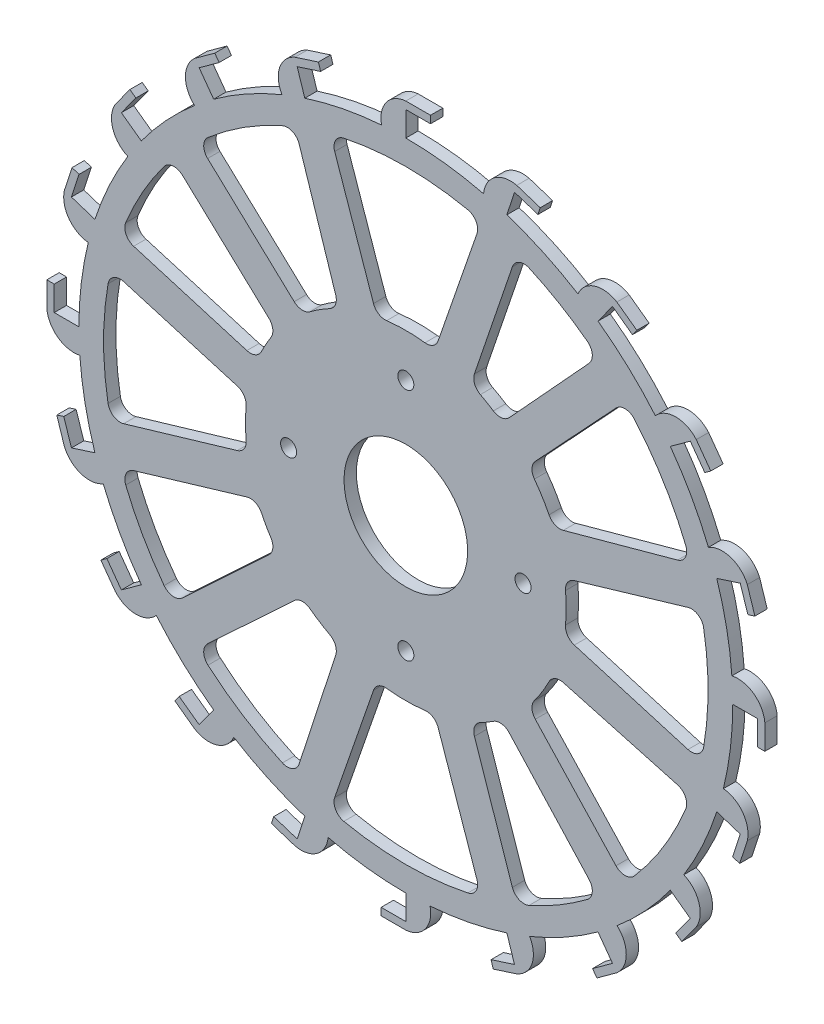
SolidWorks part; units mm, degrees
material "Q235A"
ref_plane "前视基准面" through (0, 0, 0) normal (0, 0, 1) x (1, 0, 0)
ref_plane "上视基准面" through (0, 0, 0) normal (0, 1, 0) x (1, 0, 0)
ref_plane "右视基准面" through (0, 0, 0) normal (1, 0, 0) x (0, 0, -1)
sketch "草图1" plane through (0, 0, 0) normal (0, 0, 1) x (1, 0, 0)
  line B0 (115.4655, -40.9141) -> (25.2954, -16.1289)
  line B1 (88.8732, -84.3078) -> (25.2954, -16.1289)
  line B2 (-30.6464, 118.6046) -> (-11.7362, 63.9317)
  line B3 (30.6464, 118.6046) -> (11.7362, 63.9317)
  line B4 (-119.6013, -26.4909) -> (-64.2083, -10.1138)
  line B5 (-119.6013, 26.4909) -> (-64.2083, 10.1138)
  line B6 (30.6464, -118.6046) -> (11.7362, -63.9317)
  line B7 (-30.6464, -118.6046) -> (-11.7362, -63.9317)
  line B8 (-115.4672, 40.9094) -> (-26.3476, 14.3458)
  line B9 (-94.5377, 77.903) -> (-26.3476, 14.3458)
  line B10 (-94.5377, -77.903) -> (-26.3476, -14.3458)
  line B11 (-115.4672, -40.9094) -> (-26.3476, -14.3458)
  line B12 (-44.9165, -113.9682) -> (-16.1091, -25.3081)
  line B13 (-84.3077, -88.8733) -> (-16.1091, -25.3081)
  line B14 (77.9043, -94.5366) -> (15, -25.9808)
  line B15 (44.9136, -113.9694) -> (15, -25.9808)
  line B16 (88.8732, 84.3078) -> (25.2954, 16.1289)
  line B17 (115.4655, 40.9141) -> (25.2954, 16.1289)
  line B18 (119.6013, 26.4909) -> (64.2083, 10.1138)
  line B19 (119.6013, -26.4909) -> (64.2083, -10.1138)
  line B20 (44.9136, 113.9694) -> (15, 25.9808)
  line B21 (77.9043, 94.5366) -> (15, 25.9808)
  line B22 (-84.3077, 88.8733) -> (-16.1091, 25.3081)
  line B23 (-44.9165, 113.9682) -> (-16.1091, 25.3081)
  line B24 (0, 145.5) -> (10, 145.5)
  line B25 (10, 145.5) -> (10, 142.5)
  line B26 (10, 142.5) -> (0, 142.5)
  line B27 (0, 132.5) -> (0, 142.5)
  line B28 (-44.962, 138.3787) -> (-35.4514, 141.4689)
  line B29 (-35.4514, 141.4689) -> (-34.5244, 138.6157)
  line B30 (-34.5244, 138.6157) -> (-44.0349, 135.5256)
  line B31 (-40.9448, 126.015) -> (-44.0349, 135.5256)
  line B32 (-85.5228, 117.712) -> (-77.4326, 123.5898)
  line B33 (-77.4326, 123.5898) -> (-75.6692, 121.1628)
  line B34 (-75.6692, 121.1628) -> (-83.7594, 115.2849)
  line B35 (-77.8815, 107.1948) -> (-83.7594, 115.2849)
  line B36 (-117.712, 85.5228) -> (-111.8341, 93.6129)
  line B37 (-111.8341, 93.6129) -> (-109.4071, 91.8496)
  line B38 (-109.4071, 91.8496) -> (-115.2849, 83.7594)
  line B39 (-107.1948, 77.8815) -> (-115.2849, 83.7594)
  line B40 (-138.3787, 44.962) -> (-135.2886, 54.4725)
  line B41 (-135.2886, 54.4725) -> (-132.4354, 53.5455)
  line B42 (-132.4354, 53.5455) -> (-135.5256, 44.0349)
  line B43 (-126.015, 40.9448) -> (-135.5256, 44.0349)
  line B44 (-145.5, 0) -> (-145.5, 10)
  line B45 (-145.5, 10) -> (-142.5, 10)
  line B46 (-142.5, 10) -> (-142.5, 0)
  line B47 (-132.5, 0) -> (-142.5, 0)
  line B48 (-138.3787, -44.962) -> (-141.4689, -35.4514)
  line B49 (-141.4689, -35.4514) -> (-138.6157, -34.5244)
  line B50 (-138.6157, -34.5244) -> (-135.5256, -44.0349)
  line B51 (-126.015, -40.9448) -> (-135.5256, -44.0349)
  line B52 (-117.712, -85.5228) -> (-123.5898, -77.4326)
  line B53 (-123.5898, -77.4326) -> (-121.1628, -75.6692)
  line B54 (-121.1628, -75.6692) -> (-115.2849, -83.7594)
  line B55 (-107.1948, -77.8815) -> (-115.2849, -83.7594)
  line B56 (-85.5228, -117.712) -> (-93.6129, -111.8341)
  line B57 (-93.6129, -111.8341) -> (-91.8496, -109.4071)
  line B58 (-91.8496, -109.4071) -> (-83.7594, -115.2849)
  line B59 (-77.8815, -107.1948) -> (-83.7594, -115.2849)
  line B60 (-44.962, -138.3787) -> (-54.4725, -135.2886)
  line B61 (-54.4725, -135.2886) -> (-53.5455, -132.4354)
  line B62 (-53.5455, -132.4354) -> (-44.0349, -135.5256)
  line B63 (-40.9448, -126.015) -> (-44.0349, -135.5256)
  line B64 (0, -145.5) -> (-10, -145.5)
  line B65 (-10, -145.5) -> (-10, -142.5)
  line B66 (-10, -142.5) -> (0, -142.5)
  line B67 (0, -132.5) -> (0, -142.5)
  line B68 (44.962, -138.3787) -> (35.4514, -141.4689)
  line B69 (35.4514, -141.4689) -> (34.5244, -138.6157)
  line B70 (34.5244, -138.6157) -> (44.0349, -135.5256)
  line B71 (40.9448, -126.015) -> (44.0349, -135.5256)
  line B72 (85.5228, -117.712) -> (77.4326, -123.5898)
  line B73 (77.4326, -123.5898) -> (75.6692, -121.1628)
  line B74 (75.6692, -121.1628) -> (83.7594, -115.2849)
  line B75 (77.8815, -107.1948) -> (83.7594, -115.2849)
  line B76 (117.712, -85.5228) -> (111.8341, -93.6129)
  line B77 (111.8341, -93.6129) -> (109.4071, -91.8496)
  line B78 (109.4071, -91.8496) -> (115.2849, -83.7594)
  line B79 (107.1948, -77.8815) -> (115.2849, -83.7594)
  line B80 (138.3787, -44.962) -> (135.2886, -54.4725)
  line B81 (135.2886, -54.4725) -> (132.4354, -53.5455)
  line B82 (132.4354, -53.5455) -> (135.5256, -44.0349)
  line B83 (126.015, -40.9448) -> (135.5256, -44.0349)
  line B84 (145.5, 0) -> (145.5, -10)
  line B85 (145.5, -10) -> (142.5, -10)
  line B86 (142.5, -10) -> (142.5, 0)
  line B87 (132.5, 0) -> (142.5, 0)
  line B88 (138.3787, 44.962) -> (141.4689, 35.4514)
  line B89 (141.4689, 35.4514) -> (138.6157, 34.5244)
  line B90 (138.6157, 34.5244) -> (135.5256, 44.0349)
  line B91 (126.015, 40.9448) -> (135.5256, 44.0349)
  line B92 (117.712, 85.5228) -> (123.5898, 77.4326)
  line B93 (123.5898, 77.4326) -> (121.1628, 75.6692)
  line B94 (121.1628, 75.6692) -> (115.2849, 83.7594)
  line B95 (107.1948, 77.8815) -> (115.2849, 83.7594)
  line B96 (85.5228, 117.712) -> (93.6129, 111.8341)
  line B97 (93.6129, 111.8341) -> (91.8496, 109.4071)
  line B98 (91.8496, 109.4071) -> (83.7594, 115.2849)
  line B99 (77.8815, 107.1948) -> (83.7594, 115.2849)
  line B100 (44.962, 138.3787) -> (54.4725, 135.2886)
  line B101 (54.4725, 135.2886) -> (53.5455, 132.4354)
  line B102 (53.5455, 132.4354) -> (44.0349, 135.5256)
  line B103 (40.9448, 126.015) -> (44.0349, 135.5256)
  arc B104 (88.8732, -84.3078) -> (115.4655, -40.9141) centre (0, 0) ccw
  arc B105 (30.6464, 118.6046) -> (-30.6464, 118.6046) centre (0, 0) ccw
  arc B106 (-119.6013, 26.4909) -> (-119.6013, -26.4909) centre (0, 0) ccw
  arc B107 (-30.6464, -118.6046) -> (30.6464, -118.6046) centre (0, 0) ccw
  arc B108 (-94.5377, 77.903) -> (-115.4672, 40.9094) centre (0, 0) ccw
  arc B109 (-115.4672, -40.9094) -> (-94.5377, -77.903) centre (0, 0) ccw
  arc B110 (-84.3077, -88.8733) -> (-44.9165, -113.9682) centre (0, 0) ccw
  arc B111 (44.9136, -113.9694) -> (77.9043, -94.5366) centre (0, 0) ccw
  arc B112 (115.4655, 40.9141) -> (88.8732, 84.3078) centre (0, 0) ccw
  arc B113 (119.6013, -26.4909) -> (119.6013, 26.4909) centre (0, 0) ccw
  arc B114 (77.9043, 94.5366) -> (44.9136, 113.9694) centre (0, 0) ccw
  arc B115 (-44.9165, 113.9682) -> (-84.3077, 88.8733) centre (0, 0) ccw
  circle B116 centre (0, 0) radius 15
  arc B117 (-9.8137, 132.1361) -> (-40.9448, 126.015) centre (0, 0) ccw
  arc B118 (-50.1657, 122.6363) -> (-77.8815, 107.1948) centre (0, 0) ccw
  arc B119 (-85.6071, 101.132) -> (-107.1948, 77.8815) centre (0, 0) ccw
  arc B120 (-112.6687, 69.7282) -> (-126.015, 40.9448) centre (0, 0) ccw
  arc B121 (-128.7015, 31.4989) -> (-132.5, 0) centre (0, 0) ccw
  arc B122 (-132.1361, -9.8137) -> (-126.015, -40.9448) centre (0, 0) ccw
  arc B123 (-122.6363, -50.1657) -> (-107.1948, -77.8815) centre (0, 0) ccw
  arc B124 (-101.132, -85.6071) -> (-77.8815, -107.1948) centre (0, 0) ccw
  arc B125 (-69.7282, -112.6687) -> (-40.9448, -126.015) centre (0, 0) ccw
  arc B126 (-31.4989, -128.7015) -> (0, -132.5) centre (0, 0) ccw
  arc B127 (9.8137, -132.1361) -> (40.9448, -126.015) centre (0, 0) ccw
  arc B128 (50.1657, -122.6363) -> (77.8815, -107.1948) centre (0, 0) ccw
  arc B129 (85.6071, -101.132) -> (107.1948, -77.8815) centre (0, 0) ccw
  arc B130 (112.6687, -69.7282) -> (126.015, -40.9448) centre (0, 0) ccw
  arc B131 (128.7015, -31.4989) -> (132.5, 0) centre (0, 0) ccw
  arc B132 (132.1361, 9.8137) -> (126.015, 40.9448) centre (0, 0) ccw
  arc B133 (122.6363, 50.1657) -> (107.1948, 77.8815) centre (0, 0) ccw
  arc B134 (101.132, 85.6071) -> (77.8815, 107.1948) centre (0, 0) ccw
  arc B135 (69.7282, 112.6687) -> (40.9448, 126.015) centre (0, 0) ccw
  arc B136 (31.4989, 128.7015) -> (0, 132.5) centre (0, 0) ccw
  arc B137 (0, 145.5) -> (-9.8137, 132.1361) centre (0.9207, 134.5386) ccw
  arc B138 (-44.962, 138.3787) -> (-50.1657, 122.6363) centre (-40.6991, 128.2383) ccw
  arc B139 (-85.5228, 117.712) -> (-85.6071, 101.132) centre (-78.3349, 109.3852) ccw
  arc B140 (-117.712, 85.5228) -> (-112.6687, 69.7282) centre (-108.3028, 79.8247) ccw
  arc B141 (-138.3787, 44.962) -> (-128.7015, 31.4989) centre (-127.6693, 42.4504) ccw
  arc B142 (-145.5, 0) -> (-132.1361, -9.8137) centre (-134.5386, 0.9207) ccw
  arc B143 (-138.3787, -44.962) -> (-122.6363, -50.1657) centre (-128.2383, -40.6991) ccw
  arc B144 (-117.712, -85.5228) -> (-101.132, -85.6071) centre (-109.3852, -78.3349) ccw
  arc B145 (-85.5228, -117.712) -> (-69.7282, -112.6687) centre (-79.8247, -108.3028) ccw
  arc B146 (-44.962, -138.3787) -> (-31.4989, -128.7015) centre (-42.4504, -127.6693) ccw
  arc B147 (0, -145.5) -> (9.8137, -132.1361) centre (-0.9207, -134.5386) ccw
  arc B148 (44.962, -138.3787) -> (50.1657, -122.6363) centre (40.6991, -128.2383) ccw
  arc B149 (85.5228, -117.712) -> (85.6071, -101.132) centre (78.3349, -109.3852) ccw
  arc B150 (117.712, -85.5228) -> (112.6687, -69.7282) centre (108.3028, -79.8247) ccw
  arc B151 (138.3787, -44.962) -> (128.7015, -31.4989) centre (127.6693, -42.4504) ccw
  arc B152 (145.5, 0) -> (132.1361, 9.8137) centre (134.5386, -0.9207) ccw
  arc B153 (138.3787, 44.962) -> (122.6363, 50.1657) centre (128.2383, 40.6991) ccw
  arc B154 (117.712, 85.5228) -> (101.132, 85.6071) centre (109.3852, 78.3349) ccw
  arc B155 (85.5228, 117.712) -> (69.7282, 112.6687) centre (79.8247, 108.3028) ccw
  arc B156 (44.962, 138.3787) -> (31.4989, 128.7015) centre (42.4504, 127.6693) ccw
  arc B157 (-64.2083, 10.1138) -> (-64.2083, -10.1138) centre (0, 0) ccw
  arc B158 (-11.7362, -63.9317) -> (11.7362, -63.9317) centre (0, 0) ccw
  arc B159 (11.7362, 63.9317) -> (-11.7362, 63.9317) centre (0, 0) ccw
  arc B160 (64.2083, -10.1138) -> (64.2083, 10.1138) centre (0, 0) ccw
  circle B161 centre (47.5, 0) radius 3.25
  circle B162 centre (0, -47.5) radius 3.25
  circle B163 centre (-47.5, 0) radius 3.25
  circle B164 centre (0, 47.5) radius 3.25
sketch_block_instance "转片2-1"
sketch_block "转片2"
extrude "凸台-拉伸1" add sketch "草图1" along normal blind 5
sketch "草图2" plane through (0, 0, 5) normal (0, 0, 1) x (1, 0, 0)
  line L0 (-84.3077, 88.8733) -> (-16.1091, 25.3081) construction
  line L1 (-16.1091, 25.3081) -> (-44.9165, 113.9682) construction
  line L2 (-115.4672, 40.9094) -> (-26.3476, 14.3458) construction
  line L3 (-26.3476, 14.3458) -> (-94.5377, 77.903) construction
  line L4 (-42.0947, 49.5282) -> (-16.1091, 25.3081)
  line L5 (-16.1091, 25.3081) -> (-27.0849, 59.0882)
  line L6 (-60.2284, 24.4446) -> (-26.3476, 14.3458)
  line L7 (-26.3476, 14.3458) -> (-52.327, 38.5601)
  line L8 (15, -25.9808) -> (44.9136, -113.9694) construction
  line L9 (77.9043, -94.5366) -> (15, -25.9808) construction
  line L10 (25.2954, -16.1289) -> (88.8732, -84.3078) construction
  line L11 (115.4655, -40.9141) -> (25.2954, -16.1289) construction
  line L12 (25.2954, 16.1289) -> (115.4655, 40.9141) construction
  line L13 (88.8732, 84.3078) -> (25.2954, 16.1289) construction
  line L14 (15, 25.9808) -> (77.9043, 94.5366) construction
  line L15 (44.9136, 113.9694) -> (15, 25.9808) construction
  line L16 (15, -25.9808) -> (26.3658, -59.4125)
  line L17 (38.9255, -52.0558) -> (15, -25.9808)
  line L18 (25.2954, -16.1289) -> (49.519, -42.1055)
  line L19 (59.747, -25.5987) -> (25.2954, -16.1289)
  line L20 (25.2954, 16.1289) -> (59.747, 25.5987)
  line L21 (49.519, 42.1055) -> (25.2954, 16.1289)
  line L22 (15, 25.9808) -> (38.9255, 52.0558)
  line L23 (26.3658, 59.4125) -> (15, 25.9808)
  line L24 (-26.3476, -14.3458) -> (-115.4672, -40.9094) construction
  line L25 (-94.5377, -77.903) -> (-26.3476, -14.3458) construction
  line L26 (-16.1091, -25.3081) -> (-84.3077, -88.8733) construction
  line L27 (-44.9165, -113.9682) -> (-16.1091, -25.3081) construction
  line L28 (-26.3476, -14.3458) -> (-60.2284, -24.4446)
  line L29 (-52.327, -38.5601) -> (-26.3476, -14.3458)
  line L30 (-16.1091, -25.3081) -> (-42.0947, -49.5282)
  line L31 (-27.0849, -59.0882) -> (-16.1091, -25.3081)
  arc A0 (-27.0849, 59.0882) -> (-42.0947, 49.5282) centre (0, 0) ccw
  arc A1 (38.9255, 52.0558) -> (26.3658, 59.4125) centre (0, 0) ccw
  arc A2 (59.747, 25.5987) -> (49.519, 42.1055) centre (0, 0) ccw
  arc A3 (49.519, -42.1055) -> (59.747, -25.5987) centre (0, 0) ccw
  arc A4 (26.3658, -59.4125) -> (38.9255, -52.0558) centre (0, 0) ccw
  arc A5 (-42.0947, -49.5282) -> (-27.0849, -59.0882) centre (0, 0) ccw
  arc A6 (-60.2284, -24.4446) -> (-52.327, -38.5601) centre (0, 0) ccw
  arc A7 (-52.327, 38.5601) -> (-60.2284, 24.4446) centre (0, 0) ccw
extrude "凸台-拉伸3" add sketch "草图2" against normal through all
fillet "圆角1" radius 5 48 edges at (59.747, -25.5987, 2.5) (49.519, -42.1055, 2.5) (88.8732, -84.3078, 2.5) (115.4655, -40.9141, 2.5) (-11.7362, 63.9317, 2.5) (11.7362, 63.9317, 2.5) (30.6464, 118.6046, 2.5) (-30.6464, 118.6046, 2.5) (-64.2083, -10.1138, 2.5) (-64.2083, 10.1138, 2.5) (-119.6013, 26.4909, 2.5) (-119.6013, -26.4909, 2.5) (11.7362, -63.9317, 2.5) (-11.7362, -63.9317, 2.5) (-30.6464, -118.6046, 2.5) (30.6464, -118.6046, 2.5) (-60.2284, 24.4446, 2.5) (-52.327, 38.5601, 2.5) (-94.5377, 77.903, 2.5) (-52.327, -38.5601, 2.5) (-60.2284, -24.4446, 2.5) (-115.4672, -40.9094, 2.5) (-94.5377, -77.903, 2.5) (-27.0849, -59.0882, 2.5) (-42.0947, -49.5282, 2.5) (-84.3077, -88.8733, 2.5) (-44.9165, -113.9682, 2.5) (38.9255, -52.0558, 2.5) (26.3658, -59.4125, 2.5) (44.9136, -113.9694, 2.5) (77.9043, -94.5366, 2.5) (49.519, 42.1055, 2.5) (59.747, 25.5987, 2.5) (115.4655, 40.9141, 2.5) (88.8732, 84.3078, 2.5) (64.2083, 10.1138, 2.5) (64.2083, -10.1138, 2.5) (119.6013, -26.4909, 2.5) (119.6013, 26.4909, 2.5) (26.3658, 59.4125, 2.5) (38.9255, 52.0558, 2.5) (77.9043, 94.5366, 2.5) (44.9136, 113.9694, 2.5) (-42.0947, 49.5282, 2.5) (-27.0849, 59.0882, 2.5) (-44.9165, 113.9682, 2.5) (-84.3077, 88.8733, 2.5) (-115.4672, 40.9094, 2.5)
sketch "草图3" plane through (0, 0, 0) normal (0, 0, -1) x (-1, 0, 0)
  circle A0 centre (0, 0) radius 25.05
  dimension "D1" = 50.1
extrude "切除-拉伸1" cut sketch "草图3" against normal through all
